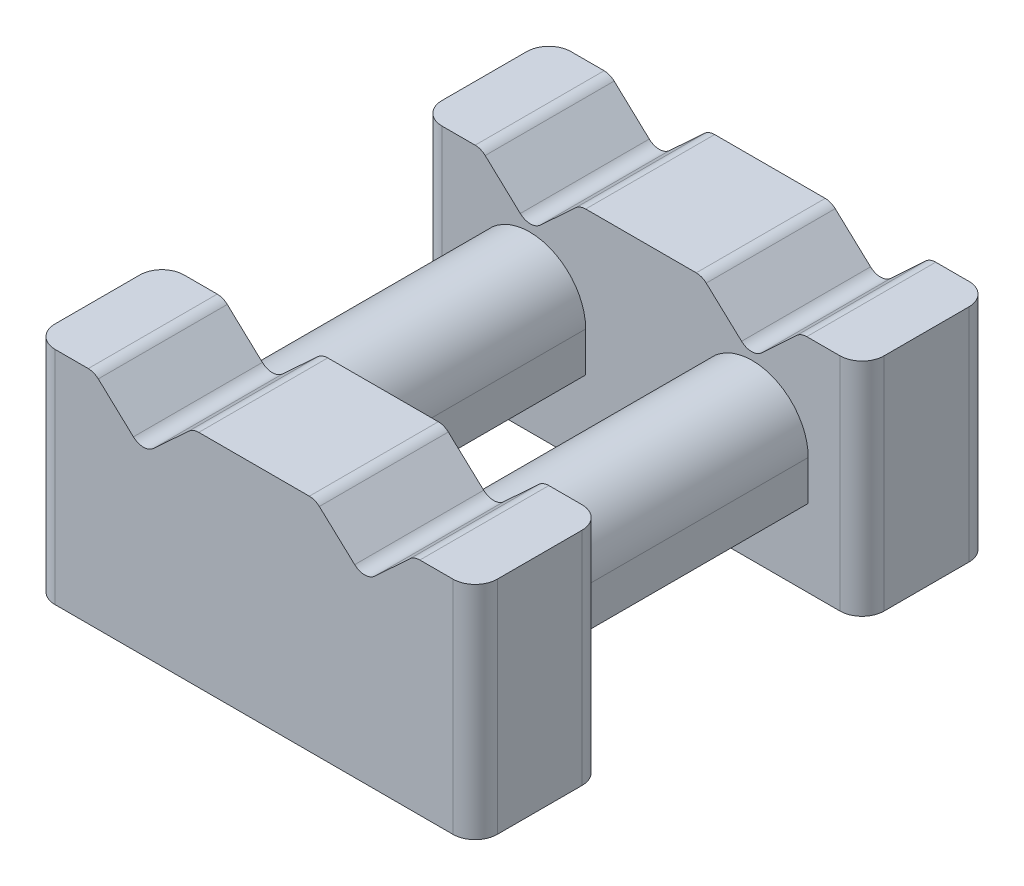
from build123d import *

# Parameters (mm, degrees)
SKETCH_1_W          = 6
SKETCH_1_H          = 3
EXTRUDE_1_DEPTH     = 1.75
EXTRUDE_2_DEPTH     = 3.5
FILLET_5_R          = 0.3
FILLET_6_R          = 0.3
FILLET_7_R          = 0.3
FILLET_8_R          = 0.3
SKETCH_6_W          = 6
SKETCH_6_H          = 3
EXTRUDE_4_DEPTH     = 1.75
FILLET_9_R          = 0.3
FILLET_10_R         = 0.3
FILLET_11_R         = 0.3
FILLET_12_R         = 0.3
CUT_EXTRUDE_1_DEPTH = 10.300192295


with BuildPart() as part:
    # 草图1 → 凸台-拉伸1 (new body)
    with BuildSketch(Plane.XY):
        with Locations((-0.722891566, 3.361445783)):
            Rectangle(SKETCH_1_W, SKETCH_1_H)
    extrude(amount=EXTRUDE_1_DEPTH)

    # 草图2 → 凸台-拉伸2 (add)
    with BuildSketch(Plane(origin=(0, 0, 0), x_dir=(-1, 0, 0), z_dir=(0, 0, -1))):
        with BuildLine():
            Line((-0.097402615, 2.911445783), (-0.027108434, 2.911445783))
            Line((-0.027108434, 2.911445783), (-0.027108434, 3.451445783))
            ThreePointArc((-0.027108434, 3.451445783), (-0.787108434, 4.211445783), (-1.547108434, 3.451445783))
            Line((-1.547108434, 3.451445783), (-1.547108434, 2.911445783))
            Line((-1.547108434, 2.911445783), (-1.456814252, 2.911445783))
            ThreePointArc((-1.456814252, 2.911445783), (-0.777108434, 2.491445783), (-0.097402615, 2.911445783))
        make_face()
        with BuildLine():
            Line((1.472891566, 3.451445783), (1.472891566, 2.911445783))
            Line((1.472891566, 2.911445783), (1.543185748, 2.911445783))
            ThreePointArc((1.543185748, 2.911445783), (2.222891566, 2.491445783), (2.902597385, 2.911445783))
            Line((2.902597385, 2.911445783), (2.992891566, 2.911445783))
            Line((2.992891566, 2.911445783), (2.992891566, 3.451445783))
            ThreePointArc((2.992891566, 3.451445783), (2.232891566, 4.211445783), (1.472891566, 3.451445783))
        make_face()
    extrude(amount=EXTRUDE_2_DEPTH)

    # 圆角5
    fillet_5_edges = [part.edges().sort_by_distance(p)[0] for p in [
        (2.277108434, 3.361445783, 1.75),
    ]]
    fillet(fillet_5_edges, radius=FILLET_5_R)

    # 圆角6
    fillet_6_edges = [part.edges().sort_by_distance(p)[0] for p in [
        (2.277108434, 3.361445783, 0),
    ]]
    fillet(fillet_6_edges, radius=FILLET_6_R)

    # 圆角7
    fillet_7_edges = [part.edges().sort_by_distance(p)[0] for p in [
        (-3.722891566, 3.361445783, 1.75),
    ]]
    fillet(fillet_7_edges, radius=FILLET_7_R)

    # 圆角8
    fillet_8_edges = [part.edges().sort_by_distance(p)[0] for p in [
        (-3.722891566, 3.361445783, 0),
    ]]
    fillet(fillet_8_edges, radius=FILLET_8_R)

    # 草图6 → 凸台-拉伸4 (add)
    with BuildSketch(Plane(origin=(0, 0, -3.5), x_dir=(-1, 0, 0), z_dir=(0, 0, -1))):
        with Locations((0.722891566, 3.361445783)):
            Rectangle(SKETCH_6_W, SKETCH_6_H)
    extrude(amount=EXTRUDE_4_DEPTH)

    # 圆角9
    fillet_9_edges = [part.edges().sort_by_distance(p)[0] for p in [
        (2.277108434, 3.361445783, -5.25),
    ]]
    fillet(fillet_9_edges, radius=FILLET_9_R)

    # 圆角10
    fillet_10_edges = [part.edges().sort_by_distance(p)[0] for p in [
        (2.277108434, 3.361445783, -3.5),
    ]]
    fillet(fillet_10_edges, radius=FILLET_10_R)

    # 圆角11
    fillet_11_edges = [part.edges().sort_by_distance(p)[0] for p in [
        (-3.722891566, 3.361445783, -5.25),
    ]]
    fillet(fillet_11_edges, radius=FILLET_11_R)

    # 圆角12
    fillet_12_edges = [part.edges().sort_by_distance(p)[0] for p in [
        (-3.722891566, 3.361445783, -3.5),
    ]]
    fillet(fillet_12_edges, radius=FILLET_12_R)

    # 草图7 → 切除-拉伸1 (cut, through all)
    with BuildSketch(Plane.XY.offset(1.75)):
        with BuildLine():
            Line((-2.972891566, 4.861445783), (-1.472891566, 4.861445783))
            ThreePointArc((-1.472891566, 4.861445783), (-1.545812961, 4.847678085), (-1.608694758, 4.808270485))
            Line((-1.608694758, 4.808270485), (-2.088349842, 4.364621081))
            ThreePointArc((-2.088349842, 4.364621081), (-2.224416187, 4.311445956), (-2.360342129, 4.36497896))
            Line((-2.360342129, 4.36497896), (-2.836702471, 4.807912606))
            ThreePointArc((-2.836702471, 4.807912606), (-2.899725196, 4.847581976), (-2.972891566, 4.861445783))
        make_face()
        with BuildLine():
            Line((0.162911626, 4.808270485), (0.642566709, 4.364621081))
            ThreePointArc((0.642566709, 4.364621081), (0.778633055, 4.311445956), (0.914558997, 4.36497896))
            Line((0.914558997, 4.36497896), (1.390919338, 4.807912606))
            ThreePointArc((1.390919338, 4.807912606), (1.453942064, 4.847581976), (1.527108434, 4.861445783))
            Line((1.527108434, 4.861445783), (0.027108434, 4.861445783))
            ThreePointArc((0.027108434, 4.861445783), (0.100029829, 4.847678085), (0.162911626, 4.808270485))
        make_face()
    extrude(amount=-CUT_EXTRUDE_1_DEPTH, mode=Mode.SUBTRACT)


solid = part.part
